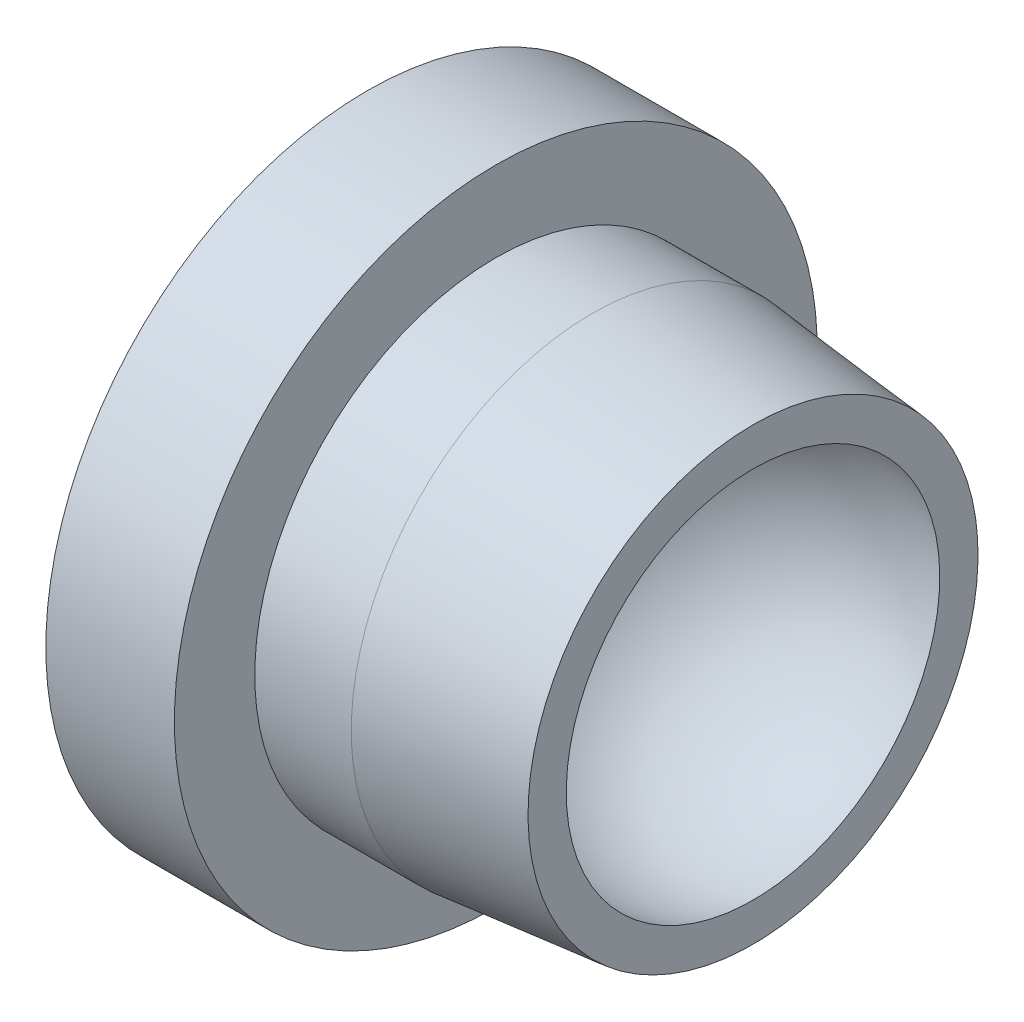
SolidWorks part; units mm, degrees
ref_plane "Front Plane" through (0, 0, 0) normal (0, 0, 1) x (1, 0, 0)
ref_plane "Top Plane" through (0, 0, 0) normal (0, 1, 0) x (1, 0, 0)
ref_plane "Right Plane" through (0, 0, 0) normal (1, 0, 0) x (0, 0, -1)
sketch "Sketch1" plane through (0, 0, 0) normal (0, 0, 1) x (1, 0, 0)
  line L0 (0, 0) -> (0, 10)
  line L1 (0, 10) -> (4, 10)
  line L2 (4, 10) -> (4, 7.5)
  line L3 (4, 7.5) -> (7, 7.5)
  line L4 (7, 7.5) -> (12, 7)
  line L5 (12, 7) -> (12, 0)
  line L6 (12, 0) -> (0, 0)
  dimension "D1" = 10
  dimension "D2" = 4
  dimension "D3" = 7
  dimension "D4" = 12
  dimension "D5" = 7.5
  dimension "D6" = 5
revolve "Revolve1" add sketch "Sketch1" angle 360 about L6
sketch "Sketch2" plane through (0, 0, 0) normal (-1, 0, 0) x (0, 0, 1)
  circle A0 centre (0, 0) radius 4
  dimension "D1" = 8
extrude "Cut-Extrude1" cut sketch "Sketch2" against normal blind 2
sketch "Sketch3" plane through (2, 0, 0) normal (-1, 0, 0) x (0, 0, 1)
  circle A0 centre (0, 0) radius 0.5
  dimension "D1" = 1
extrude "Cut-Extrude2" cut sketch "Sketch3" against normal blind 15
sketch "Sketch5" plane through (0, 0, 0) normal (-1, 0, 0) x (0, 0, 1)
  circle A0 centre (0, 0) radius 2
  dimension "D1" = 4
extrude "Cut-Extrude3" cut sketch "Sketch5" against normal blind 15 from offset 3.5 offset against normal yes
sketch "Sketch6" plane through (0, 0, 0) normal (0, 0, 1) x (1, 0, 0)
  line L0 (6.6, 0) -> (-6.6, 0) construction
  line L1 (12, -7) -> (12, 7) construction
  line L2 (4.5, 0) -> (16.5, 0)
  arc A0 (16.5, 0) -> (4.5, 0) centre (10.5, 0) ccw
  dimension "D1" = 12
  dimension "D2" = 1.5
revolve "Cut-Revolve1" cut sketch "Sketch6" angle 360 about L2
